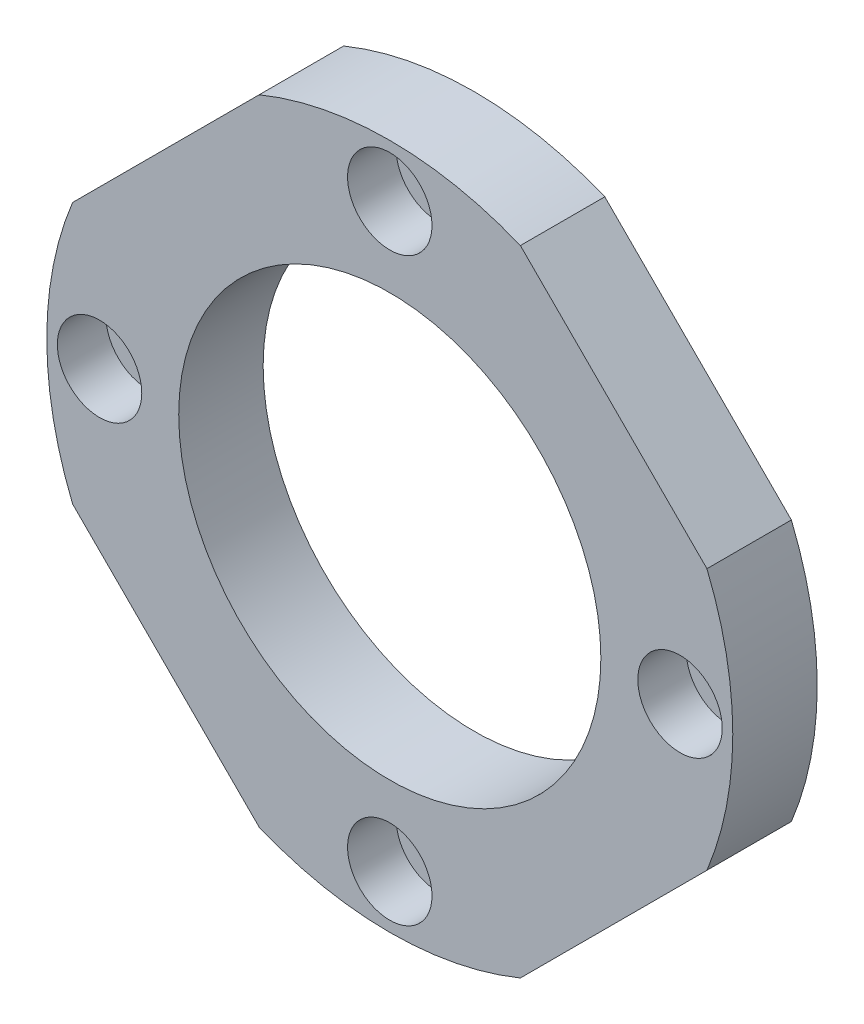
from build123d import *

# Parameters (mm, degrees)
SKETCH1_R                                            = 20
BOSS_EXTRUDE1_DEPTH                                  = 8
HOLE_SIZE_PER_SOCKET_HEAD_CAP_SCREW_TYPE_D           = 4.5
HOLE_SIZE_PER_SOCKET_HEAD_CAP_SCREW_TYPE_CBORE_D     = 8
HOLE_SIZE_PER_SOCKET_HEAD_CAP_SCREW_TYPE_CBORE_DEPTH = 4.6


with BuildPart() as part:
    # Sketch1 → Boss-Extrude1 (new body)
    with BuildSketch(Plane.XY):
        with BuildLine():
            Line((-30.0520382, -12.374368671), (-12.374368671, -30.0520382))
            ThreePointArc((-12.374368671, -30.0520382), (0, -32.5), (12.374368671, -30.0520382))
            Line((12.374368671, -30.0520382), (30.0520382, -12.374368671))
            ThreePointArc((30.0520382, -12.374368671), (32.5, 0), (30.0520382, 12.374368671))
            Line((30.0520382, 12.374368671), (12.374368671, 30.0520382))
            ThreePointArc((12.374368671, 30.0520382), (0, 32.5), (-12.374368671, 30.0520382))
            Line((-12.374368671, 30.0520382), (-30.0520382, 12.374368671))
            ThreePointArc((-30.0520382, 12.374368671), (-32.5, 0), (-30.0520382, -12.374368671))
        make_face()
        Circle(SKETCH1_R, mode=Mode.SUBTRACT)
    extrude(amount=BOSS_EXTRUDE1_DEPTH)

    # Hole size per socket head cap screw type 1 (through all)
    with Locations(Plane.XY.offset(8)):
        with Locations((0, 27.5), (-27.5, 0), (0, -27.5), (27.5, 0)):
            CounterBoreHole(HOLE_SIZE_PER_SOCKET_HEAD_CAP_SCREW_TYPE_D / 2, HOLE_SIZE_PER_SOCKET_HEAD_CAP_SCREW_TYPE_CBORE_D / 2, HOLE_SIZE_PER_SOCKET_HEAD_CAP_SCREW_TYPE_CBORE_DEPTH)


solid = part.part
